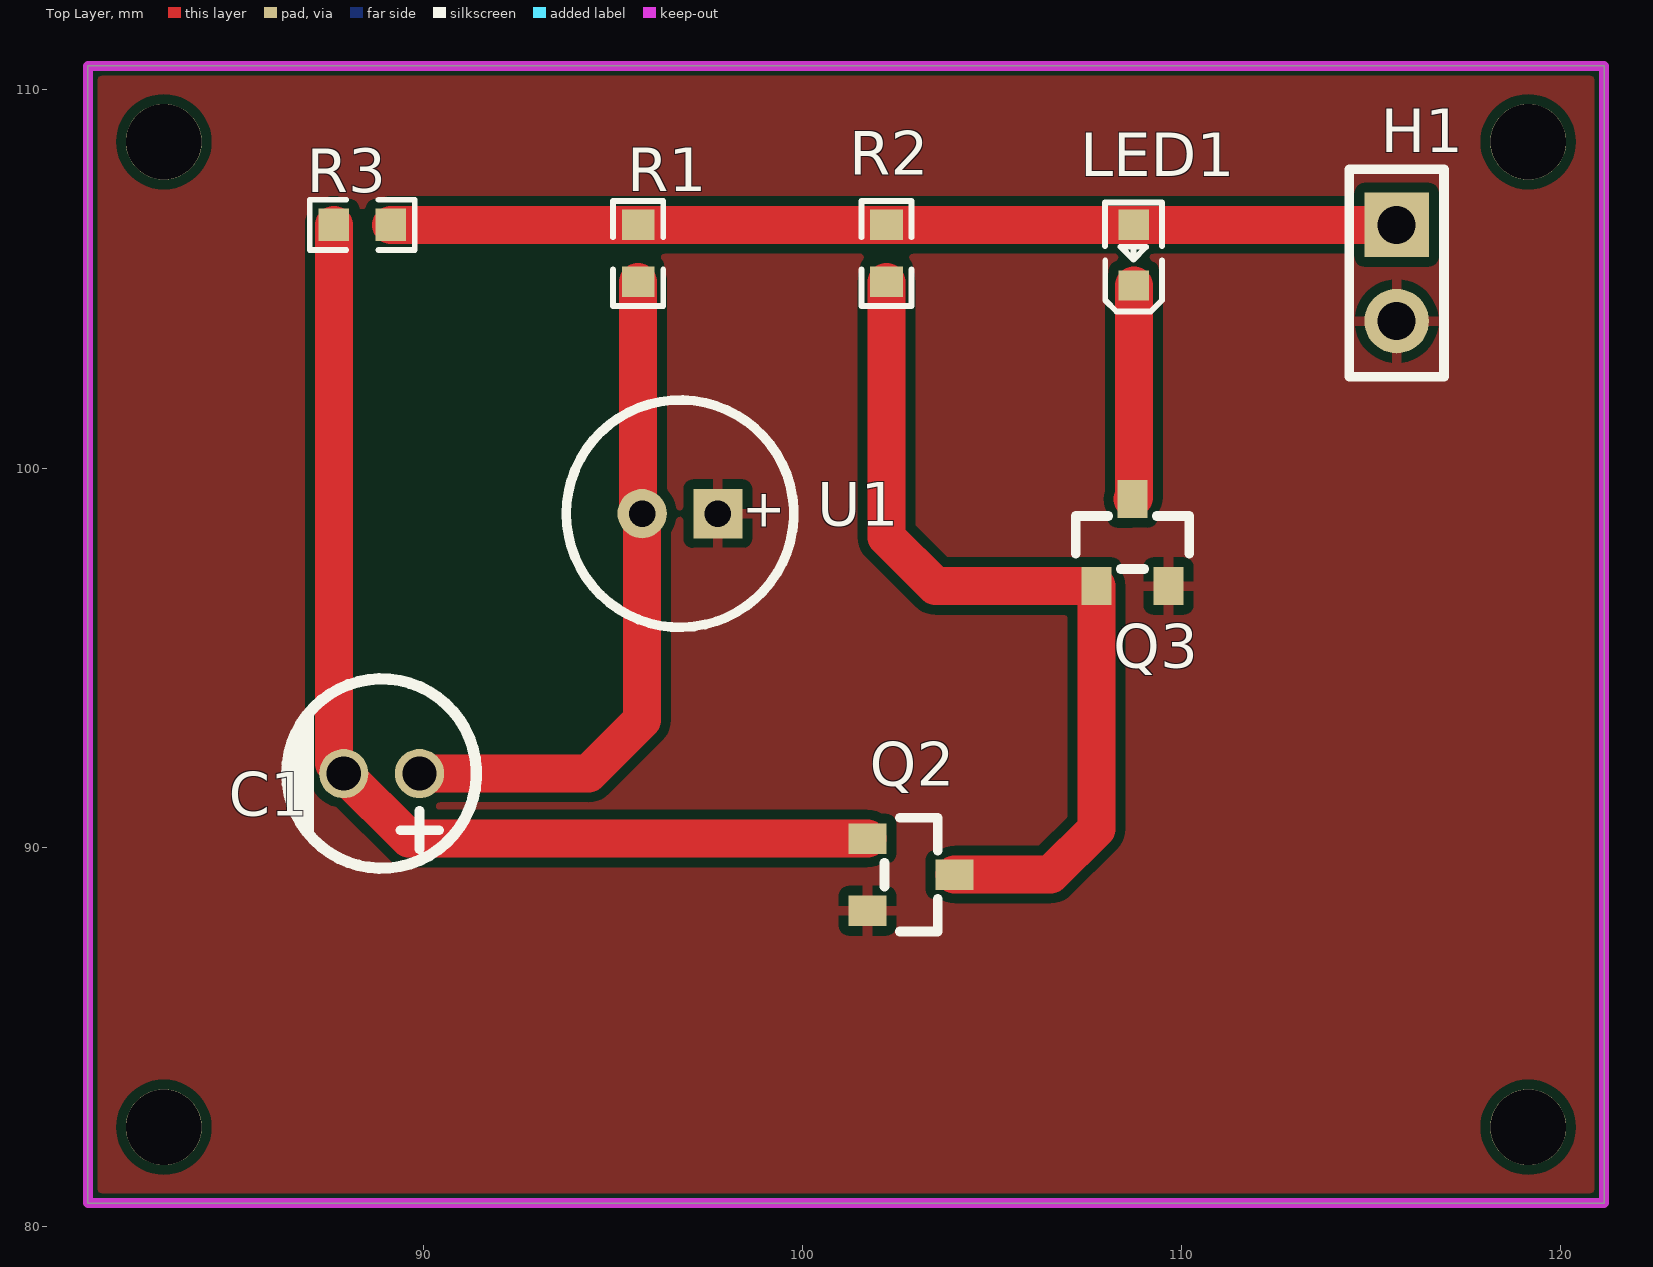
[diagram p0: Top Layer view]
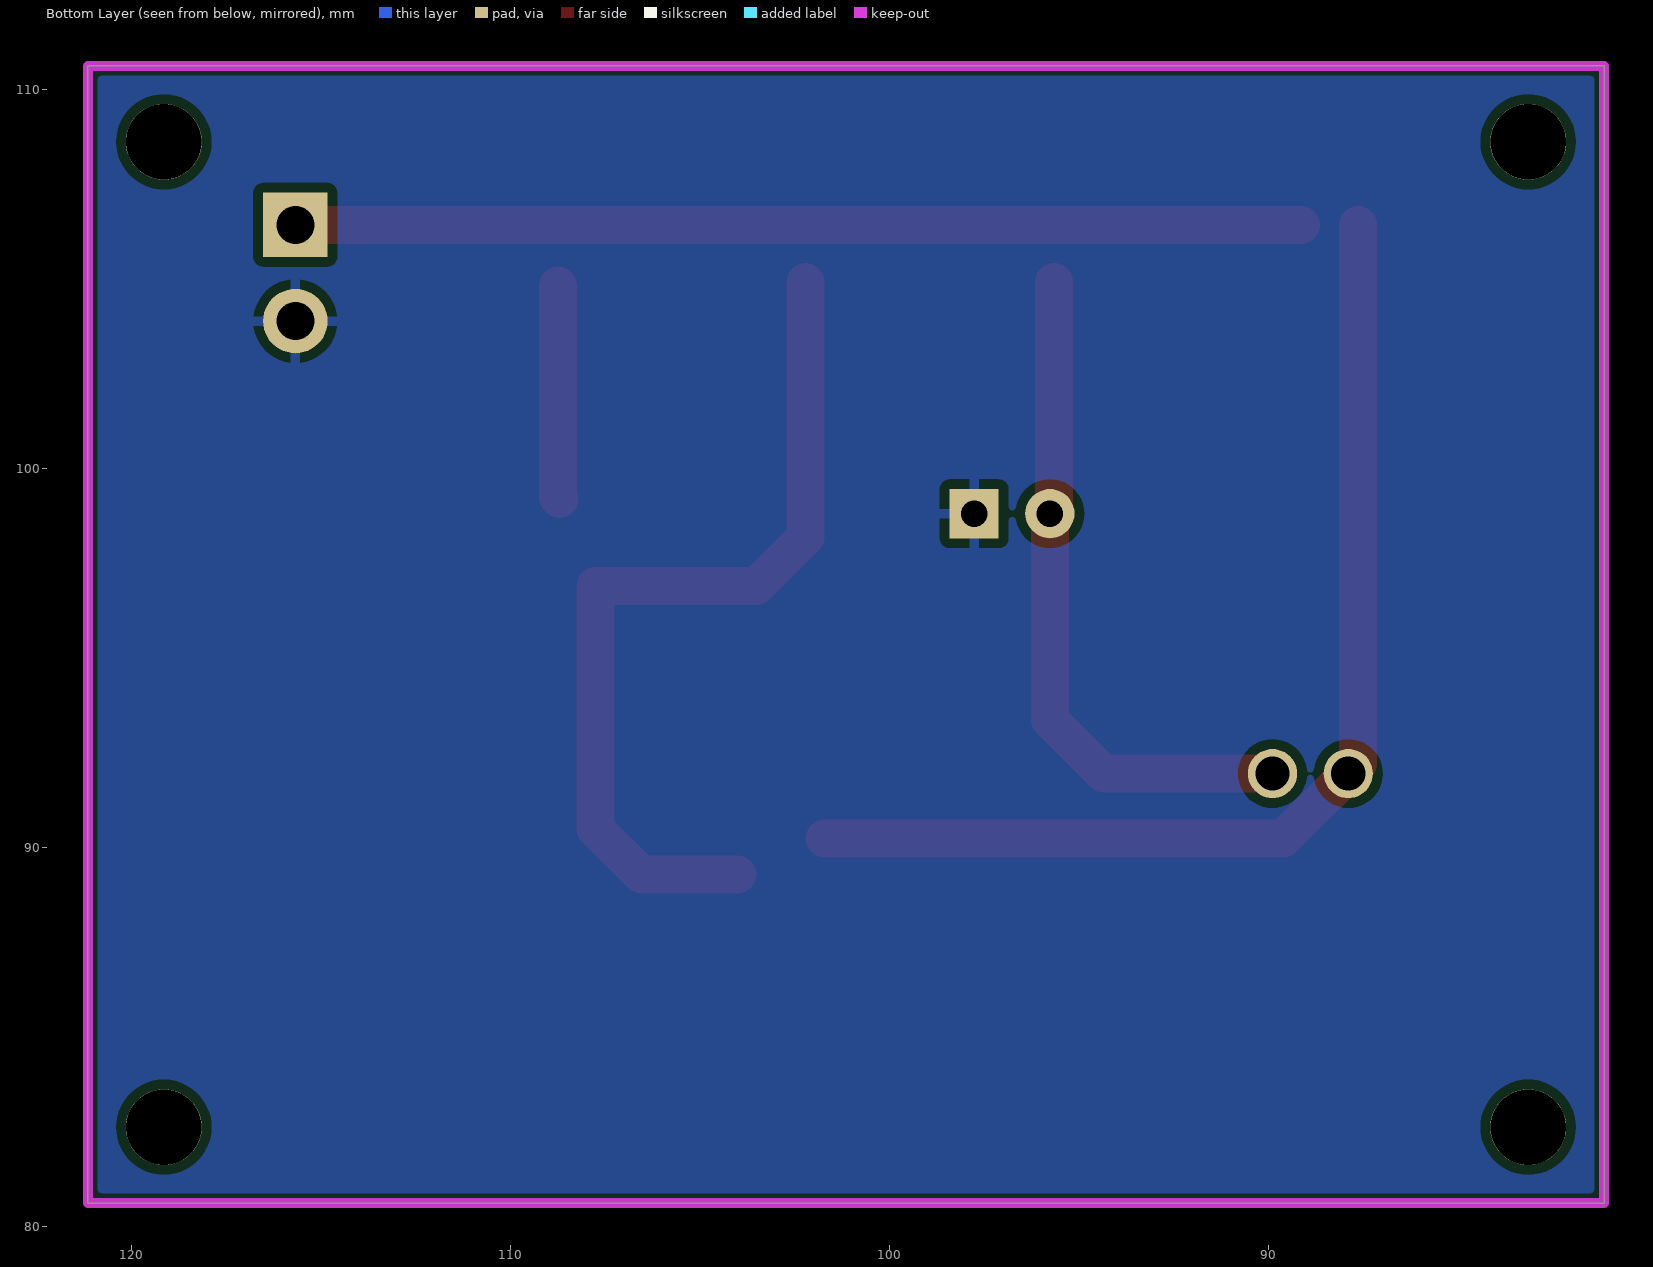
[diagram p1: Bottom Layer view, seen from below]
# Altium PCB MISC52075.pcbdoc
Units mm, origin at the board's own origin, x right, y up, seen from the top; angles counter-clockwise.
Board outline 40 x 30 mm, 2 copper layers (Top Layer, Bottom Layer), stack 1.58 mm thick; 9 components, 6 nets, 24 pads, 0 vias.

## Layer stack, top to bottom
Top Solder Mask Layer: solder mask 0.01, Dk 3.3
Top Layer: signal copper 0.035
Dielectric1: surface 1.51, FR4, Dk 4.5
Bottom Layer: signal copper 0.035
Bottom Solder Mask Layer: solder mask 0.01, Dk 3.3

## Board outline
81.153,110.617 81.153,80.617 121.153,80.617 121.153,110.617

## Design rules (kind name [scope] priority, off if disabled: settings)
BoardOutlineClearance copperThickness2oz_1 [All] p2 off: genericclearance=0.203 ignorepadtopadclearanceinfootprint=FALSE except(0: Arc-SplitContinuation Track-SplitContinuation SMDPad-SplitContinuation THPad-SplitContinuation Via-SplitContinuation Fill-SplitContinuation Region-SplitContinuation Poly-SplitContinuation Text-SplitContinuation Hole-SplitContinuation; 0.152: Arc-CutoutEdge SMDPad-CutoutEdge THPad-CutoutEdge Via-CutoutEdge Fill-CutoutEdge Region-CutoutEdge Text-CutoutEdge; 0.176: Hole-OutlineEdge Hole-CutoutEdge; 0.254: Poly-OutlineEdge Poly-CutoutEdge; 0.3: Arc-OutlineEdge Track-OutlineEdge SMDPad-OutlineEdge THPad-OutlineEdge Via-OutlineEdge Fill-OutlineEdge Region-OutlineEdge Text-OutlineEdge Track-CutoutEdge)
BoardOutlineClearance copperThickness1oz_1 [All] p4: genericclearance=0.102 ignorepadtopadclearanceinfootprint=FALSE except(0: Arc-SplitContinuation Track-SplitContinuation SMDPad-SplitContinuation THPad-SplitContinuation Via-SplitContinuation Fill-SplitContinuation Region-SplitContinuation Poly-SplitContinuation Text-SplitContinuation Hole-SplitContinuation; 0.152: SMDPad-CutoutEdge THPad-CutoutEdge Via-CutoutEdge Fill-CutoutEdge Region-CutoutEdge Text-CutoutEdge; 0.176: Hole-OutlineEdge Hole-CutoutEdge; 0.254: Poly-OutlineEdge Poly-CutoutEdge; 0.3: Arc-OutlineEdge Track-OutlineEdge SMDPad-OutlineEdge THPad-OutlineEdge Via-OutlineEdge Fill-OutlineEdge Region-OutlineEdge Text-OutlineEdge Arc-CutoutEdge Track-CutoutEdge)
Clearance copperThickness2oz [All] p1 off: gap=0.203 ignorepadtopadclearanceinfootprint=FALSE except(0.152: SMDPad-Track SMDPad-SMDPad THPad-Track SMDPad-THPad THPad-THPad Track-Via SMDPad-Via THPad-Via Via-Via Fill-Track Region-Track Fill-SMDPad Region-SMDPad Fill-THPad Region-THPad Fill-Via Region-Via Fill-Fill Fill-Region Region-Region Arc-Track Arc-SMDPad Arc-THPad Arc-Via Fill-Arc Region-Arc Arc-Arc Text-Track SMDPad-Text Text-THPad Text-Via Fill-Text Region-Text Arc-Text Text-Text; 0.176: Hole-Track Hole-SMDPad Hole-THPad Hole-Via Fill-Hole Region-Hole Hole-Arc Hole-Text; 0.254: Poly-Track Poly-SMDPad Poly-THPad Poly-Via Poly-Fill Poly-Region Poly-Poly Poly-Arc Poly-Text Poly-Hole)
Clearance copperThickness1oz [All] p3: gap=0.102 ignorepadtopadclearanceinfootprint=FALSE except(0.152: SMDPad-Track SMDPad-SMDPad THPad-Track SMDPad-THPad THPad-THPad Track-Via SMDPad-Via THPad-Via Via-Via Fill-Track Region-Track Fill-SMDPad Region-SMDPad Fill-THPad Region-THPad Fill-Via Region-Via Fill-Fill Fill-Region Region-Region Arc-Track Arc-SMDPad Arc-THPad Arc-Via Fill-Arc Region-Arc Arc-Arc Text-Track SMDPad-Text Text-THPad Text-Via Fill-Text Region-Text Arc-Text Text-Text; 0.176: Hole-Track Hole-SMDPad Hole-THPad Hole-Via Fill-Hole Region-Hole Hole-Arc Hole-Text; 0.254: Poly-Track Poly-SMDPad Poly-THPad Poly-Via Poly-Fill Poly-Region Poly-Poly Poly-Arc Poly-Text Poly-Hole)
Creepage creepage [All] p1: checkdistance=0 ignoreinternallayers=TRUE applytopolygonpour=TRUE
DiffPairsRouting differentialPair [All] p1: maxlimit=0.152 minlimit=0.152 mostfreqgap=0.152 toplayer_minwidth=0.127 toplayer_prefwidth=0.254 toplayer_maxwidth=2.54 toplayer_mingap=0.152 toplayer_prefgap=0.152 toplayer_maxgap=0.152 bottomlayer_minwidth=0.127 bottomlayer_prefwidth=0.254 bottomlayer_maxwidth=2.54 bottomlayer_mingap=0.152 bottomlayer_prefgap=0.152 bottomlayer_maxgap=0.152 maxuncoupledlength=0.254
HoleToHoleClearance otherClearance [All] p1: gap=0.3 allowstackedmicrovias=TRUE
Length netLength [All] p1: minlimit=0 maxlimit=0
MatchedLengths netLengthTolerance [All] p1: tolerance=25.4
PasteMaskExpansion pasteMaskExpansion [All] p1: expansion=0
PlaneConnect innerPlane [All] p1: planeconnectstyle=Relief reliefexpansion=0.508 reliefentries=4 reliefconductorwidth=0.254 reliefairgap=0.254
PolygonConnect copperRegion [(InNet('GND'))] p1: connectstyle=Relief reliefconductorwidth=0.254 reliefentries=4 polygonreliefangle="90 Angle" airgapwidth=0.254 via.connectstyle=Relief via.reliefconductorwidth=0.254 via.reliefentries=4 via.polygonreliefangle="90 Angle" via.airgapwidth=0.254
RoutingVias viaSize [All] p1: holewidth=0.305 width=0.61 viastyle="Through Hole" minholewidth=0.3 minwidth=0.5 maxholewidth=6.3 maxwidth=10
SolderMaskExpansion solderMaskExpansion [IsVia] p1: expansion=-25.4 istentingtop=TRUE
SolderMaskExpansion solderMaskExpansion [All] p2: expansion=0.051 istentingtop=FALSE
Width copperThickness2oz_2 [All] p1 off: maxlimit=2.54 minlimit=0.203 preferedwidth=0.254
Width copperThickness1oz_2 [All] p2: maxlimit=2.54 minlimit=0.127 preferedwidth=0.254

## Components (designator, comment, footprint, x,y, rotation, side; value= is the part's Value field where it differs from the comment)
C1 "10uF" CAP-TH_BD5.0-P2.00-D0.8-FD-10UF50VC110GL 88.9,91.948 r180 top
H1 "" HDR-TH_2P-P2.54-V-F 115.682,105.156 r270 top
LED1 "" LED_0603 108.738,105.677 r90 top
Q2 "" S8050_SOT-23 102.87,89.281 r180 top
Q3 "" S8050_SOT-23 108.712,98.044 r270 top
R1 "150K" R0603 95.67,105.673 r90 top
R2 "10K" R0603 102.222,105.673 r90 top
R3 "1M" R0603 88.392,106.426 r0 top
U1 "电流源" 咪头 96.774,98.806 r180 top

## Footprints (in the part's own frame and the unit in brackets; to place one, negate y for a bottom-side part, rotate by r counter-clockwise, add the part's x,y. Pads: shape width x height; smd on the part's side, far side on the other; paste and mask are expansions set on the pad)
CAP-TH_BD5.0-P2.00-D0.8-FD-10UF50VC110GL [mm]
  round 1.3 hole 0.9 paste+0 mask+0.051: 1(-1,0) 2(1,0)
  silkscreen extent -2.5,-2.5 2.5,2.5
HDR-TH_2P-P2.54-V-F [mm]
  rect 1.7x1.7 hole 1: 1(-1.27,0)
  round 1.7 hole 1: 2(1.27,0)
  silkscreen extent -2.74,-1.25 2.74,1.25
LED_0603 [mil]
  rect 31.5x31.5 smd paste+0 mask+2: 1(-33.5,-0.4) 2(29.5,-0.2)
  silkscreen extent -61,-30 53,30
R0603 [mm]
  rect 0.806x0.864 smd paste-100 mask+0.051: 1(-0.753,0) 2(0.753,0)
  silkscreen extent -1.39,-0.66 1.39,0.66
S8050_SOT-23 [mm]
  rect 1x0.8 smd paste+0 mask+0.051: 1(1.15,-0.95) 2(1.15,0.95) 3(-1.15,0)
  silkscreen extent -0.7,-1.5 0.7,1.5
咪头 [mm]
  rect 1.3x1.3 hole 0.7: 1(-1,0)
  round 1.3 hole 0.7: 2(1,0)
  silkscreen extent -3,-3 3,3

## Free pads (board coordinates)
  round 2 hole 2: 1(83.153,82.617) 1(83.153,108.617) 1(119.153,82.617) 1(119.153,108.617)

## Nets (pads, with @x,y where several pads share a name; then routed paths per layer and width w, separated by ;. In a path a pad name is that pad's centre, name@x,y a point inside that pad or via, vN(x,y) a via of type N, cw(c..) or ccw(c..) an arc to the next point about the centre after c; other vN are vias at no path point)
$1N6: H1.1 LED1.2 R1.2 R2.2 R3.2 | length 26.5
  Top Layer w1: R3.2 R1.2 R2.2 LED1.2 H1.1
$1N7: Q2.3 Q3.1 R2.1 | length 23.5
  Top Layer w1: R2.1 102.222,98.184 103.512,96.894 Q3.1 107.762,90.49 106.553,89.281 Q2.3
$1N9: C1.2 Q2.1 R3.1 | length 29.1
  Top Layer w1: R3.1 87.639,92.209 C1.2 89.617,90.231 Q2.1
$1N10: C1.1 R1.1 U1.2 | length 18.1
  Top Layer w1: C1.1 94.361,91.948 95.774,93.361 U1.2 95.67,98.91 R1.1
$1N15: LED1.1 Q3.3 | length 5.6
  Top Layer w1: Q3.3 108.748,99.23 LED1.1
GND: H1.2 Q2.2 Q3.2 U1.1

## Polygon pours and split planes (outlines as drawn)
GND on Top Layer (solid, remove dead copper, pour order 0): 77.597,113.157 77.597,76.2 126.238,76.2 126.238,113.157
GND on Bottom Layer (solid, remove dead copper, pour order 2): 76.2,112.649 76.2,76.327 126.365,76.327 126.365,112.649

## Keep-outs
Board Outline Layer:
  the board outline again, w0.254